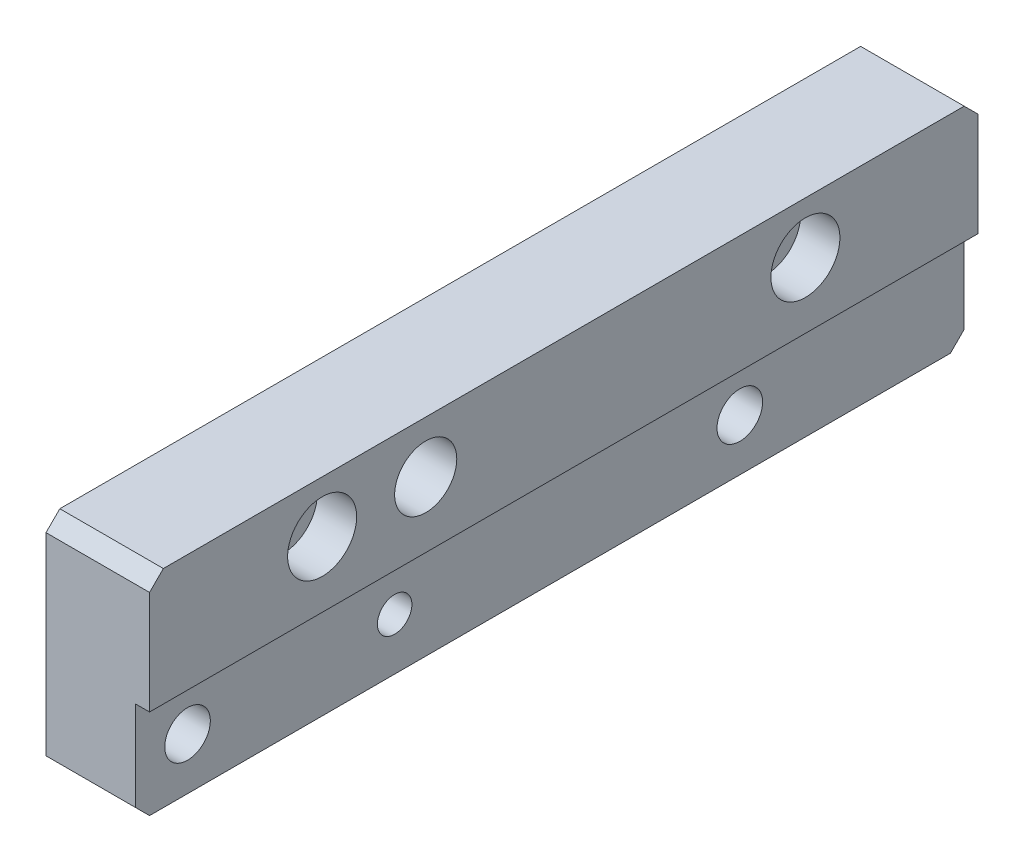
SolidWorks part; units mm, degrees
material "45#"
ref_plane "Front Plane" through (0, 0, 0) normal (0, 0, 1) x (1, 0, 0)
ref_plane "Top Plane" through (0, 0, 0) normal (0, 1, 0) x (1, 0, 0)
ref_plane "Right Plane" through (0, 0, 0) normal (1, 0, 0) x (0, 0, -1)
sketch "Sketch1" plane through (0, 0, 0) normal (1, 0, 0) x (0, 0, -1)
  line L1 (-60, -16) -> (60, -16)
  line L2 (-60, -16) -> (-60, 16)
  line L3 (-60, 16) -> (60, 16)
  line L4 (60, -16) -> (60, 16)
  line L5 (-60, -16) -> (60, 16) construction
  line L6 (-60, 16) -> (60, -16) construction
  point P0 (0, 0)
  dimension "D1" = 120
  dimension "D2" = 32
extrude "Boss-Extrude1" add sketch "Sketch1" along normal blind 15
sketch "Sketch2" plane through (15, 0, 0) normal (1, 0, 0) x (0, 0, -1)
  line L1 (-60, -16) -> (60, -16)
  line L2 (-60, -16) -> (-60, -1)
  line L3 (-60, -1) -> (60, -1)
  line L4 (60, -16) -> (60, -1)
  line L5 (-60, -16) -> (60, -16) construction
  line L6 (60, -16) -> (60, 16) construction
  line L7 (-60, 16) -> (-60, -16) construction
  dimension "D1" = 15
extrude "Cut-Extrude1" cut sketch "Sketch2" against normal blind 2
hole_wizard "Ø8.0mm blind hole 1" positions "Sketch3" profile "Sketch4" hole size "Ø8.0" standard "GB"
sketch "Sketch3" plane through (0, 0, 0) normal (-1, 0, 0) x (0, 0, 1)
  line L0 (60, 8.5) -> (-60, 8.5) construction
  line L1 (60, 16) -> (60, -16) construction
  line L2 (-60, -16) -> (-60, 16) construction
  line L4 (-60, 16) -> (60, 16) construction
  point P0 (35, 8.5)
  point P2 (-35, 8.5)
  dimension "D1" = 7.5
  dimension "D2" = 70
  dimension "D3" = 25
sketch "Sketch4" plane through (0, 8.5, 35) normal (0, 1, 0) x (0, 0, 1)
  line L0 (0, 0) -> (0, 8.4034)
  line L1 (0, 8.4034) -> (4, 6)
  line L2 (4, 6) -> (4, 0)
  line L5 (4, 0) -> (0, 0)
  line L10 (0, 8.4034) -> (-4, 6) construction
  line L11 (0, -6.35) -> (0, 107.95) construction
  dimension "孔直径" = 8
  dimension "孔深度" = 6
  dimension "导头角度" = 118
hole_wizard "M8 Clearance Hole1" positions "Sketch7" profile "Sketch8" hole size "M8" standard "GB" end condition through all
sketch "Sketch7" plane through (15, 0, 0) normal (1, 0, 0) x (0, 0, -1)
  line L0 (-35, 8.5) -> (35, 8.5) construction
  point P7 (-20, 8.5)
  dimension "D1" = 15
sketch "Sketch8" plane through (15, 8.5, 20) normal (0, 1, 0) x (0, 0, -1)
  line L0 (0, 0) -> (0, 15)
  line L1 (0, 15) -> (4.5, 15)
  line L2 (4.5, 15) -> (4.5, 0)
  line L5 (4.5, 0) -> (0, 0)
  line L11 (0, -6.35) -> (0, 107.95) construction
  dimension "通孔孔直径" = 9
  dimension "通孔孔深度" = 15
chamfer "Chamfer1" distance 2 angle 45 4 edges at (6.5, -16, -60) (7.5, 16, -60) (6.5, -16, 60) (7.5, 16, 60)
hole_wizard "CBORE for M5 Hexagon socket head cap screws1" positions "Sketch9" profile "Sketch10" counterbore size "M5" standard "GB" end condition through all
sketch "Sketch9" plane through (15, 0, 0) normal (1, 0, 0) x (0, 0, -1)
  point P0 (-35, 8.5)
  point P3 (35, 8.5)
sketch "Sketch10" plane through (15, 8.5, 35) normal (0, 1, 0) x (0, 0, -1)
  line L0 (0, 0) -> (0, 15)
  line L1 (0, 15) -> (2.75, 15)
  line L3 (2.75, 15) -> (2.75, 5.7)
  line L4 (2.75, 5.7) -> (5, 5.7)
  line L5 (5, 5.7) -> (5, 0)
  line L7 (5, 0) -> (0, 0)
  line L11 (0, -6.35) -> (0, 107.95) construction
  dimension "通孔孔直径" = 5.5
  dimension "通孔孔深度" = 15
  dimension "柱形沉头孔直径" = 10
  dimension "柱形沉头孔深度" = 5.7
hole_wizard "CBORE for M6 Hexagon socket head cap screws1" positions "Sketch11" profile "Sketch12" counterbore size "M6" standard "GB" end condition through all
sketch "Sketch11" plane through (0, 0, 0) normal (-1, 0, 0) x (0, 0, 1)
  point P0 (-27.5, -8.5)
  point P3 (52.5, -8.5)
sketch "Sketch12" plane through (0, -8.5, -27.5) normal (0, 1, 0) x (0, 0, 1)
  line L0 (0, 0) -> (0, 15)
  line L1 (0, 15) -> (3.3, 15)
  line L3 (3.3, 15) -> (3.3, 6.8)
  line L4 (3.3, 6.8) -> (5.5, 6.8)
  line L5 (5.5, 6.8) -> (5.5, 0)
  line L7 (5.5, 0) -> (0, 0)
  line L11 (0, -6.35) -> (0, 107.95) construction
  dimension "通孔孔直径" = 6.6
  dimension "通孔孔深度" = 15
  dimension "柱形沉头孔直径" = 11
  dimension "柱形沉头孔深度" = 6.8
hole_wizard "Ø5.0mm blind hole 1" positions "Sketch13" profile "Sketch14" hole size "Ø5.0" standard "GB" end condition through all
sketch "Sketch13" plane through (0, 0, 0) normal (-1, 0, 0) x (0, 0, 1)
  point P3 (22.5, -8.5)
sketch "Sketch14" plane through (0, -8.5, 22.5) normal (0, 1, 0) x (0, 0, 1)
  line L0 (0, 0) -> (0, 15)
  line L1 (0, 15) -> (2.5, 15)
  line L2 (2.5, 15) -> (2.5, 0)
  line L5 (2.5, 0) -> (0, 0)
  line L11 (0, -6.35) -> (0, 107.95) construction
  dimension "通孔孔直径" = 5
  dimension "通孔孔深度" = 15
